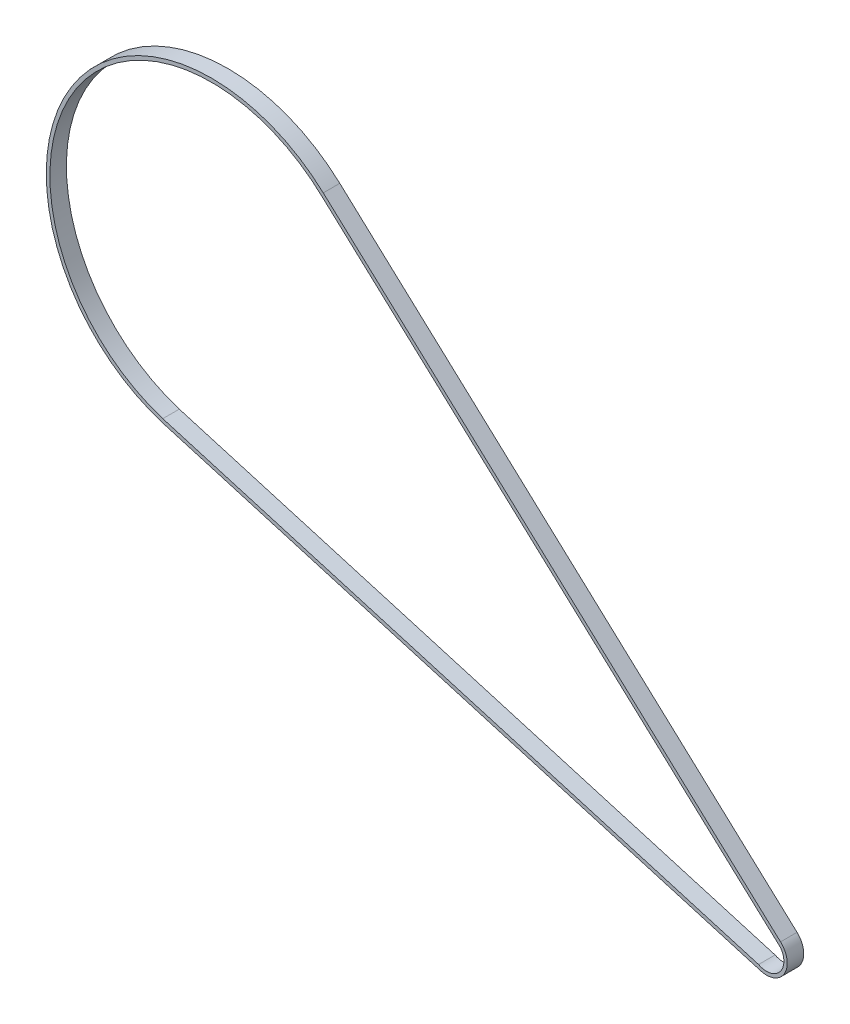
SolidWorks part; units mm, degrees
ref_plane "Front Plane" through (0, 0, 0) normal (0, 0, 1) x (1, 0, 0)
ref_plane "Top Plane" through (0, 0, 0) normal (0, 1, 0) x (1, 0, 0)
ref_plane "Right Plane" through (0, 0, 0) normal (1, 0, 0) x (0, 0, -1)
sketch "Sketch1" plane through (0, 0, 0) normal (0, 0, 1) x (1, 0, 0)
  line B0 (-460.524, 638.2055) -> (92.9759, 129.8134)
  line B1 (-652.1229, 298.9994) -> (69.026, 87.4126)
  arc B2 (-460.524, 638.2055) -> (-652.1229, 298.9994) centre (-595.816, 490.9096) ccw
  arc B3 (69.026, 87.4126) -> (92.9759, 129.8134) centre (76.0644, 111.4014) ccw
sketch_block_instance "Block 2-1-1"
sketch_block "Block 2-1"
ref_plane "Plane1" through (-460.524, 0, 0) normal (1, 0, 0) x (0, 0, -1)
sketch "Sketch2" plane through (-460.524, 0, 0) normal (1, 0, 0) x (0, 0, -1)
  line L0 (0, 733.6209) -> (0, 572.2884) construction
  line L1 (0, 638.2055) -> (74.9269, 638.2055) construction
  line L3 (-10, 638.2055) -> (10, 638.2055)
  line L4 (-10, 638.2055) -> (-10, 632.2055)
  line L5 (-10, 632.2055) -> (10, 632.2055)
  line L6 (10, 638.2055) -> (10, 632.2055)
  dimension "D1" = 20
  dimension "D2" = 6
sweep "Sweep1" add profiles "Sketch2" path "Sketch1"
